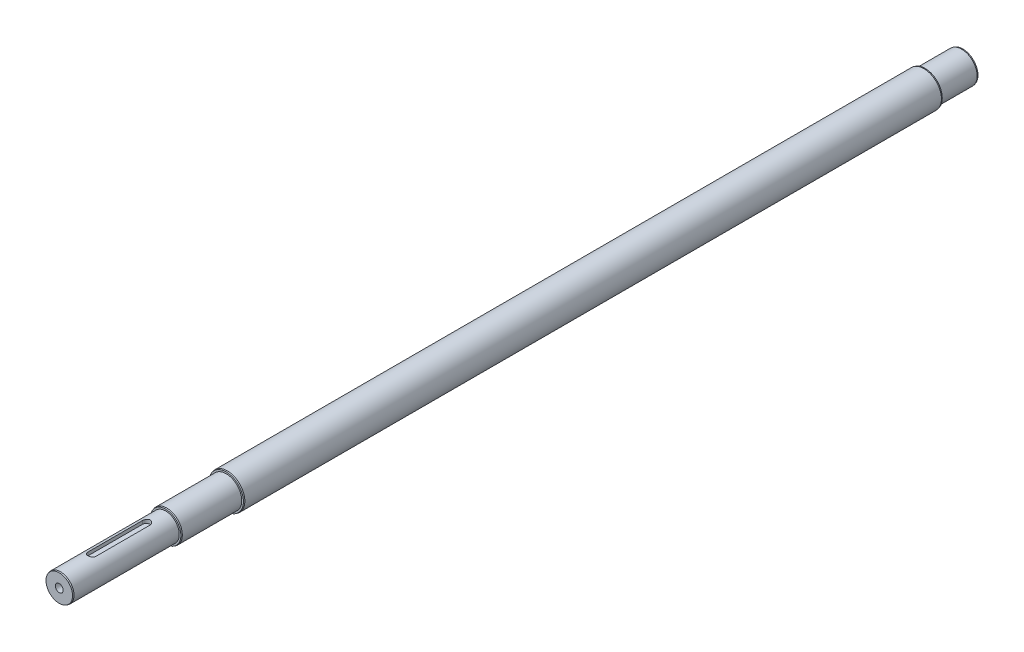
from build123d import *
from OCP.BRepFilletAPI import BRepFilletAPI_MakeChamfer

# Parameters (mm, degrees)
SKETCH_1_R              = 22.5
EXTRUDE_1_DEPTH         = 900
SKETCH_2_R              = 20
EXTRUDE_2_DEPTH         = 78
SKETCH_3_R              = 17.5
EXTRUDE_3_DEPTH         = 137
EXTRUDE_START           = 48.5
SKETCH_4_R              = 20
EXTRUDE_4_DEPTH         = 48.5
CHAMFER_1_SIZE          = 1.5
CHAMFER_1_SIZE2         = 0.401923789
CUT_EXTRUDE_1_DEPTH     = 5
HOLE_WIZARD_M12_1_D     = 10.2
HOLE_WIZARD_M12_1_DEPTH = 29.25
HOLE_WIZARD_M12_1_TIP   = 3.064389157
HOLE_WIZARD_M10_1_D     = 8.5
HOLE_WIZARD_M10_1_DEPTH = 24.5
HOLE_WIZARD_M10_1_TIP   = 2.553657631
CHAMFER_2_SIZE          = 1.5
CHAMFER_2_SIZE2         = 0.401923789
FILLET_1_R              = 1


with BuildPart() as part:
    # 草图1 → 凸台-拉伸1 (new body)
    with BuildSketch(Plane.XY):
        Circle(SKETCH_1_R)
    extrude(amount=EXTRUDE_1_DEPTH)

    # 草图2 → 凸台-拉伸2 (add)
    with BuildSketch(Plane.XY.offset(900)):
        Circle(SKETCH_2_R)
    extrude(amount=EXTRUDE_2_DEPTH)

    # 草图3 → 凸台-拉伸3 (add)
    with BuildSketch(Plane.XY.offset(978)):
        Circle(SKETCH_3_R)
    extrude(amount=EXTRUDE_3_DEPTH)

    # 草图4 → 凸台-拉伸4 (add)
    with BuildSketch(Plane(origin=(0, 0, 0), x_dir=(-1, 0, 0), z_dir=(0, 0, -1)).offset(EXTRUDE_START)):
        with Locations(Location((0, 0, 0), (0, 0, 180))):
            Circle(SKETCH_4_R)
    extrude(amount=-EXTRUDE_4_DEPTH)

    # 倒角1: one chamfer whose edges measure the first distance from different faces: ONE call of the kernel's chamfer builder (chamfer() names one face for all edges)
    chamfer_1_edges_1 = [part.edges().sort_by_distance(p)[0] for p in [
        (-17.5, 0, 1115),
    ]]
    chamfer_1_side_1 = [part.faces().sort_by_distance(p)[0] for p in [
        (-17.5, 0, 1046.5),
    ]]
    chamfer_1_edges_2 = [part.edges().sort_by_distance(p)[0] for p in [
        (-20, 0, -48.5),
    ]]
    chamfer_1_side_2 = [part.faces().sort_by_distance(p)[0] for p in [
        (-20, 0, -24.25),
    ]]
    chamfer_1_edges_3 = [part.edges().sort_by_distance(p)[0] for p in [
        (-22.5, 0, 900),
    ]]
    chamfer_1_side_3 = [part.faces().sort_by_distance(p)[0] for p in [
        (-22.5, 0, 450),
    ]]
    chamfer_1_edges_4 = [part.edges().sort_by_distance(p)[0] for p in [
        (-20, 0, 978),
    ]]
    chamfer_1_side_4 = [part.faces().sort_by_distance(p)[0] for p in [
        (-20, 0, 939),
    ]]
    chamfer_1 = BRepFilletAPI_MakeChamfer(part.part.solid().wrapped)
    for e in chamfer_1_edges_1:
        chamfer_1.Add(CHAMFER_1_SIZE, CHAMFER_1_SIZE2, e.wrapped, chamfer_1_side_1[0].wrapped)  # the first distance lies on this face
    for e in chamfer_1_edges_2:
        chamfer_1.Add(CHAMFER_1_SIZE, CHAMFER_1_SIZE2, e.wrapped, chamfer_1_side_2[0].wrapped)  # the first distance lies on this face
    for e in chamfer_1_edges_3:
        chamfer_1.Add(CHAMFER_1_SIZE, CHAMFER_1_SIZE2, e.wrapped, chamfer_1_side_3[0].wrapped)  # the first distance lies on this face
    for e in chamfer_1_edges_4:
        chamfer_1.Add(CHAMFER_1_SIZE, CHAMFER_1_SIZE2, e.wrapped, chamfer_1_side_4[0].wrapped)  # the first distance lies on this face
    add(Compound.cast(chamfer_1.Shape()), mode=Mode.REPLACE)

    # 草图5 → 切除-拉伸1 (cut)
    with BuildSketch(Plane(origin=(0, 17.5, 0), x_dir=(1, 0, 0), z_dir=(0, 1, 0))):
        with BuildLine():
            Line((5, -1003), (5, -1073))
            ThreePointArc((5, -1073), (0, -1078), (-5, -1073))
            Line((-5, -1073), (-5, -1003))
            ThreePointArc((-5, -1003), (0, -998), (5, -1003))
        make_face()
    extrude(amount=-CUT_EXTRUDE_1_DEPTH, mode=Mode.SUBTRACT)

    # M12 螺纹孔1
    with Locations(Plane.XY.offset(1115)):
        with Locations((0, 0)):
            Hole(HOLE_WIZARD_M12_1_D / 2, depth=HOLE_WIZARD_M12_1_DEPTH)
            with Locations((0, 0, -(HOLE_WIZARD_M12_1_DEPTH + HOLE_WIZARD_M12_1_TIP / 2))):  # 118° drill point
                Cone(0, HOLE_WIZARD_M12_1_D / 2, HOLE_WIZARD_M12_1_TIP, mode=Mode.SUBTRACT)

    # M10 螺纹孔1
    with Locations(Plane(origin=(0, 0, -48.5), x_dir=(-1, 0, 0), z_dir=(0, 0, -1))):
        with Locations((0, 0)):
            Hole(HOLE_WIZARD_M10_1_D / 2, depth=HOLE_WIZARD_M10_1_DEPTH)
            with Locations((0, 0, -(HOLE_WIZARD_M10_1_DEPTH + HOLE_WIZARD_M10_1_TIP / 2))):  # 118° drill point
                Cone(0, HOLE_WIZARD_M10_1_D / 2, HOLE_WIZARD_M10_1_TIP, mode=Mode.SUBTRACT)

    # 倒角2
    chamfer_2_edges = [part.edges().sort_by_distance(p)[0] for p in [
        (-22.5, 0, 0),
    ]]
    chamfer_2_side = [part.faces().sort_by_distance(p)[0] for p in [
        (-22.5, 0, 449.25),
    ]]
    chamfer(chamfer_2_edges, length=CHAMFER_2_SIZE, length2=CHAMFER_2_SIZE2, reference=chamfer_2_side[0])

    # 圆角1
    fillet_1_edges = [part.edges().sort_by_distance(p)[0] for p in [
        (-20, 0, 0),
    ]]
    fillet(fillet_1_edges, radius=FILLET_1_R)


solid = part.part
